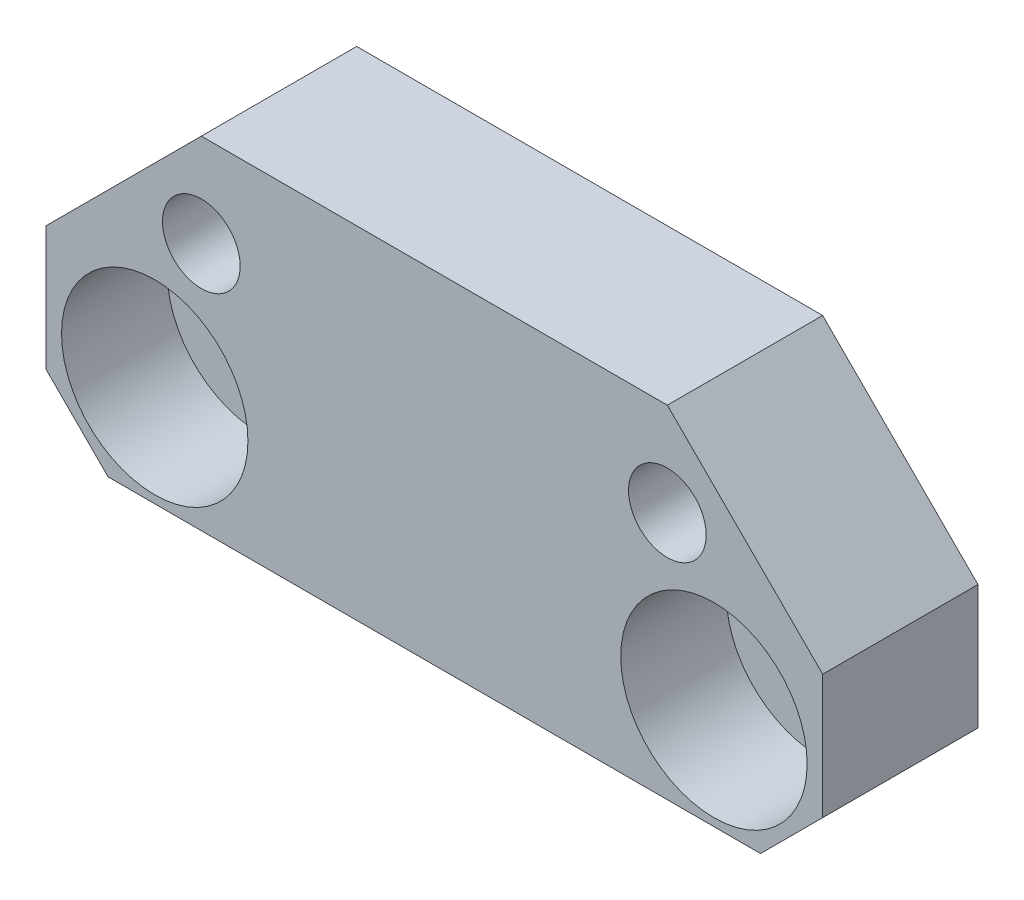
SolidWorks part; units mm, degrees
material "A6061"
ref_plane "Front Plane" through (0, 0, 0) normal (0, 0, 1) x (1, 0, 0)
ref_plane "Top Plane" through (0, 0, 0) normal (0, 1, 0) x (1, 0, 0)
ref_plane "Right Plane" through (0, 0, 0) normal (1, 0, 0) x (0, 0, -1)
sketch "Sketch1" plane through (0, 0, 0) normal (0, 0, 1) x (1, 0, 0)
  line L0 (0, 0) -> (0, -32.9084) construction
  line L1 (-12.5, -5.5) -> (12.5, -5.5)
  line L2 (-12.5, -5.5) -> (-12.5, 5.5)
  line L3 (-12.5, 5.5) -> (12.5, 5.5)
  line L4 (12.5, -5.5) -> (12.5, 5.5)
  line L5 (-12.5, -5.5) -> (12.5, 5.5) construction
  line L6 (-12.5, 5.5) -> (12.5, -5.5) construction
  line L7 (12.5, 5.5) -> (4, 5.5)
  line L8 (12.5, 5.5) -> (12.5, 2)
  line L9 (12.5, 2) -> (4, 2)
  line L10 (4, 5.5) -> (4, 2)
  line L11 (-12.5, 5.5) -> (-4, 5.5)
  line L12 (-12.5, 5.5) -> (-12.5, 2)
  line L13 (-12.5, 2) -> (-4, 2)
  line L14 (-4, 5.5) -> (-4, 2)
  point P0 (0, 0)
  dimension "D1" = 8
  dimension "D2" = 7.5
  dimension "D3" = 11
  dimension "D4" = 25
extrude "Boss-Extrude1" add sketch "Sketch1" along normal mid plane 5 contours L3 L14 L13 L2 L1 L4 L9 L10 | L3 L10 L9 L4 | L14 L3 L2 L13
hole_wizard "M3 Tapped Hole1" positions "Sketch3" profile "Sketch2" tap size "M3" standard "GB" end condition up to next
sketch "Sketch3" plane through (0, 0, 2.5) normal (0, 0, 1) x (1, 0, 0)
  line L1 (0, 0) -> (0, 8.3655) construction
  line L5 (-12.5, 5.5) -> (12.5, 5.5) construction
  point P0 (-7.5, 2.5)
  point P5 (7.5, 2.5)
  dimension "D1" = 3
  dimension "D2" = 15
sketch "Sketch2" plane through (-7.5, 2.5, 2.5) normal (1, 0, 0) x (0, -1, 0)
  line L0 (0, 0) -> (0, 5)
  line L1 (0, 5) -> (1.25, 5)
  line L2 (1.25, 5) -> (1.25, 0)
  line L5 (1.25, 0) -> (0, 0)
  line L11 (0, -6.35) -> (0, 107.95) construction
  dimension "通孔螺纹孔钻头直径" = 2.5
  dimension "通孔螺纹孔钻头深度" = 5
cosmetic thread "Hole thread1" parameters "D2"=3
cosmetic thread "Hole thread2" parameters "D2"=3
hole_wizard "Hole size (by socket head cap screw type)1" positions "Sketch5" profile "Sketch4" counterbore size "M3" standard "GB" end condition up to next
sketch "Sketch5" plane through (0, 0, 2.5) normal (0, 0, 1) x (1, 0, 0)
  line L0 (0, 0) -> (0, -17.5877) construction
  line L5 (-12.5, -5.5) -> (12.5, -5.5) construction
  point P0 (9, -2.25)
  point P3 (-9, -2.25)
  dimension "D1" = 18
  dimension "D2" = 3.25
sketch "Sketch4" plane through (9, -2.25, 2.5) normal (1, 0, 0) x (0, -1, 0)
  line L0 (0, 0) -> (0, 5)
  line L1 (0, 5) -> (1.7, 5)
  line L3 (1.7, 5) -> (1.7, 3.4)
  line L4 (1.7, 3.4) -> (3, 3.4)
  line L5 (3, 3.4) -> (3, 0)
  line L7 (3, 0) -> (0, 0)
  line L11 (0, -6.35) -> (0, 107.95) construction
  dimension "通孔孔直径" = 3.4
  dimension "通孔孔深度" = 5
  dimension "柱形沉头孔直径" = 6
  dimension "柱形沉头孔深度" = 3.4
chamfer "Chamfer2" distance 5 angle 45 2 edges at (-12.5, 5.5, 0) (12.5, 5.5, 0)
chamfer "Chamfer3" distance 2 angle 45 2 edges at (-12.5, -5.5, 0) (12.5, -5.5, 0)
